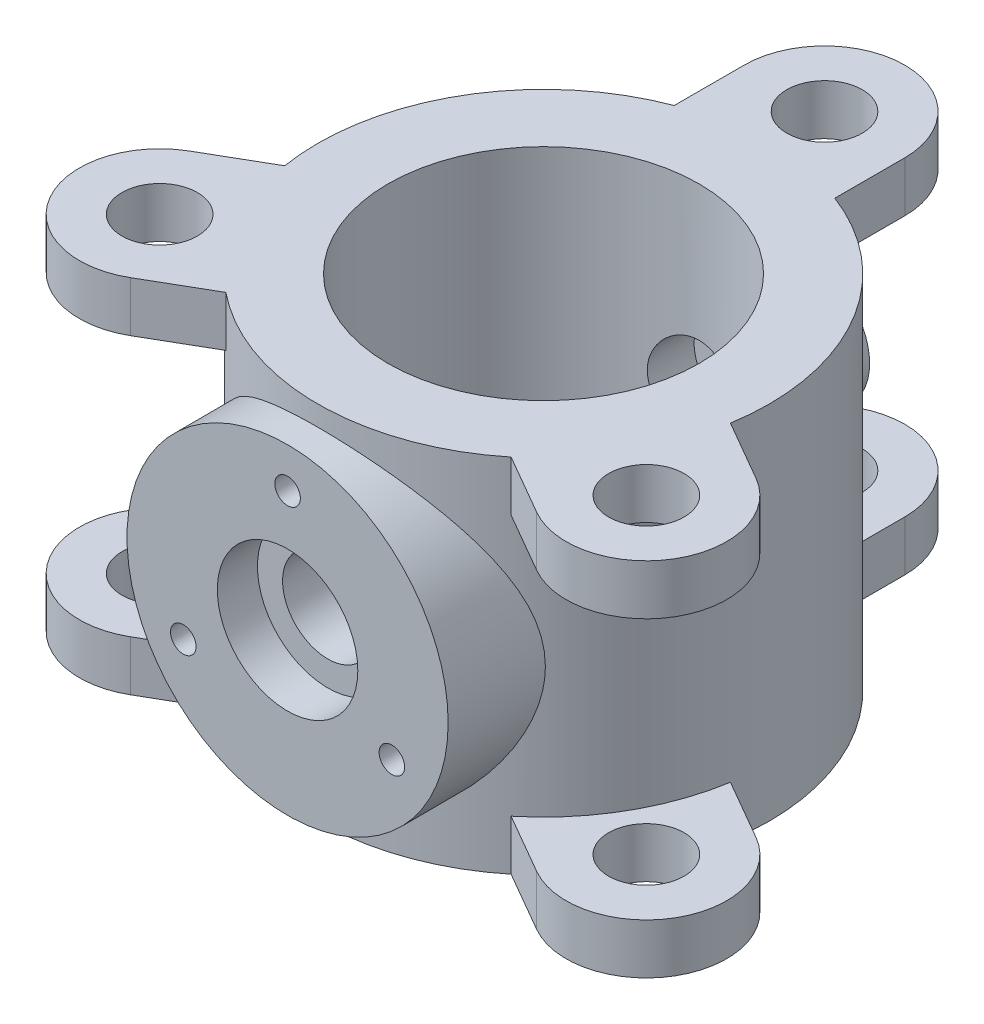
from build123d import *

# Parameters (mm, degrees)
SKETCH1_R                  = 35.7124
SKETCH1_R_2                = 24.6126
BOSS_EXTRUDE1_DEPTH        = 57.15
BOSS_EXTRUDE2_START        = -7.9502
SKETCH2_R                  = 5.969
BOSS_EXTRUDE2_DEPTH        = 7.9502
CIRPATTERN1_COUNT          = 3
MIRROR1_START              = -7.9502
MIRROR1_COPY_1_SKETCH_R    = 5.969
MIRROR1_COPY_1_DEPTH       = 7.9502
MIRROR1_COPY_2_SKETCH_R    = 5.969
MIRROR1_COPY_2_DEPTH       = 7.9502
BOSS_EXTRUDE3_REACH        = 126.178
BOSS_EXTRUDE3_END_RADIUS   = 35.7124
SKETCH3_R                  = 25.4
F_10_32_TAPPED_HOLE1_D     = 4.0386
F_10_32_TAPPED_HOLE1_DEPTH = 9.525
F_10_32_TAPPED_HOLE1_TIP   = 1.213317848
BOSS_EXTRUDE4_REACH        = 114.701
BOSS_EXTRUDE4_END_RADIUS   = 35.7124
SKETCH14_R                 = 9.525
SKETCH15_R                 = 11.1125
CUT_EXTRUDE1_DEPTH         = 6.35
SKETCH16_R                 = 7.1374
CUT_EXTRUDE2_DEPTH         = 71.4502


with BuildPart() as part:
    # Sketch1 → Boss-Extrude1 (new body)
    with BuildSketch(Plane(origin=(0, 0, 0), x_dir=(1, 0, 0), z_dir=(0, 1, 0))):
        with Locations(Location((0, 0, 0), (0, 0, 270))):
            Circle(SKETCH1_R)
        with Locations(Location((0, 0, 0), (0, 0, 270))):
            Circle(SKETCH1_R_2, mode=Mode.SUBTRACT)
    extrude(amount=BOSS_EXTRUDE1_DEPTH)

    # Sketch2 → Boss-Extrude2 (add)
    with BuildSketch(Plane(origin=(0, 57.15, 0), x_dir=(1, 0, 0), z_dir=(0, 1, 0)).offset(BOSS_EXTRUDE2_START)):
        with BuildLine():
            ThreePointArc((12.7, 44.45), (0, 57.15), (-12.7, 44.45))
            Line((-12.7, 44.45), (-12.7, 33.377919554))
            ThreePointArc((-12.7, 33.377919554), (0, 35.7124), (12.7, 33.377919554))
            Line((12.7, 33.377919554), (12.7, 44.45))
        make_face()
        with Locations(Location((0, 44.45, 0), (0, 0, 270))):
            Circle(SKETCH2_R, mode=Mode.SUBTRACT)
    boss_extrude2 = extrude(amount=BOSS_EXTRUDE2_DEPTH)

    # CirPattern1: Boss-Extrude2 ×3 about axis
    cirpattern1_axis = Axis((0, 0, 0), (0, 1, 0))
    for i in range(1, CIRPATTERN1_COUNT):
        add(boss_extrude2.rotate(cirpattern1_axis, i * 360 / CIRPATTERN1_COUNT))

    # Mirror1: Boss-Extrude2 across plane
    add(boss_extrude2.mirror(Plane.ZX.offset(28.575)))

    # Mirror1 copy 1 sketch → Mirror1 copy 1 (add)
    with BuildSketch(Plane(origin=(0, 0, 0), x_dir=(-0.4999999999999998, 0, -0.8660254037844387), z_dir=(0, -1, 0)).offset(MIRROR1_START)):
        with BuildLine():
            ThreePointArc((12.7, -44.45), (0, -57.15), (-12.7, -44.45))
            Line((-12.7, -44.45), (-12.7, -33.377919554))
            ThreePointArc((-12.7, -33.377919554), (0, -35.7124), (12.7, -33.377919554))
            Line((12.7, -33.377919554), (12.7, -44.45))
        make_face()
        with Locations((0, -44.45)):
            Circle(MIRROR1_COPY_1_SKETCH_R, mode=Mode.SUBTRACT)
    extrude(amount=MIRROR1_COPY_1_DEPTH)

    # Mirror1 copy 2 sketch → Mirror1 copy 2 (add)
    with BuildSketch(Plane(origin=(0, 0, 0), x_dir=(-0.5000000000000004, 0, 0.8660254037844384), z_dir=(0, -1, 0)).offset(MIRROR1_START)):
        with BuildLine():
            ThreePointArc((12.7, -44.45), (0, -57.15), (-12.7, -44.45))
            Line((-12.7, -44.45), (-12.7, -33.377919554))
            ThreePointArc((-12.7, -33.377919554), (0, -35.7124), (12.7, -33.377919554))
            Line((12.7, -33.377919554), (12.7, -44.45))
        make_face()
        with Locations((0, -44.45)):
            Circle(MIRROR1_COPY_2_SKETCH_R, mode=Mode.SUBTRACT)
    extrude(amount=MIRROR1_COPY_2_DEPTH)

    # Boss-Extrude3: up to this cylinder (the profile starts outside it)
    boss_extrude3_end = Plane(origin=(0, 28.575, 0), z_dir=(0, -1, 0)) * Cylinder(BOSS_EXTRUDE3_END_RADIUS, 324.7808, mode=Mode.PRIVATE)
    # Sketch3 → Boss-Extrude3 (add, up to the surface)
    with BuildSketch(Plane.XY.offset(40.4876), mode=Mode.PRIVATE) as boss_extrude3_sk1:
        with Locations((0, 28.575)):
            Circle(SKETCH3_R)
    boss_extrude3_tool1 = extrude(boss_extrude3_sk1.sketch, amount=-BOSS_EXTRUDE3_REACH, mode=Mode.PRIVATE) - boss_extrude3_end
    add(boss_extrude3_tool1.solids().sort_by_distance((0, 28.575, 40.4876))[0])

    # #10-32 Tapped Hole1
    with Locations(Plane.XY.offset(40.4876)):
        with Locations((0, 47.625), (16.497783942, 19.05), (-16.497783942, 19.05)):
            Hole(F_10_32_TAPPED_HOLE1_D / 2, depth=F_10_32_TAPPED_HOLE1_DEPTH)
            with Locations((0, 0, -(F_10_32_TAPPED_HOLE1_DEPTH + F_10_32_TAPPED_HOLE1_TIP / 2))):  # 118° drill point
                Cone(0, F_10_32_TAPPED_HOLE1_D / 2, F_10_32_TAPPED_HOLE1_TIP, mode=Mode.SUBTRACT)

    # Boss-Extrude4: up to this cylinder (the profile starts outside it)
    boss_extrude4_end = Plane(origin=(0, 28.575, 0), z_dir=(0, -1, 0)) * Cylinder(BOSS_EXTRUDE4_END_RADIUS, 301.8268, mode=Mode.PRIVATE)
    # Sketch14 → Boss-Extrude4 (add, up to the surface)
    with BuildSketch(Plane.XY.offset(-42.0624), mode=Mode.PRIVATE) as boss_extrude4_sk1:
        with Locations(Location((0, 28.575, 0), (0, 0, 90))):
            Circle(SKETCH14_R)
    boss_extrude4_tool1 = extrude(boss_extrude4_sk1.sketch, amount=BOSS_EXTRUDE4_REACH, mode=Mode.PRIVATE) - boss_extrude4_end
    add(boss_extrude4_tool1.solids().sort_by_distance((0, 28.575, -42.0624))[0])

    # Sketch15 → Cut-Extrude1 (cut)
    with BuildSketch(Plane.XY.offset(40.4876)):
        with Locations((0, 28.575)):
            Circle(SKETCH15_R)
    extrude(amount=-CUT_EXTRUDE1_DEPTH, mode=Mode.SUBTRACT)

    # Sketch16 → Cut-Extrude2 (cut)
    with BuildSketch(Plane.XY.offset(40.4876)):
        with Locations((0, 28.575)):
            Circle(SKETCH16_R)
    extrude(amount=-CUT_EXTRUDE2_DEPTH, mode=Mode.SUBTRACT)


solid = part.part
